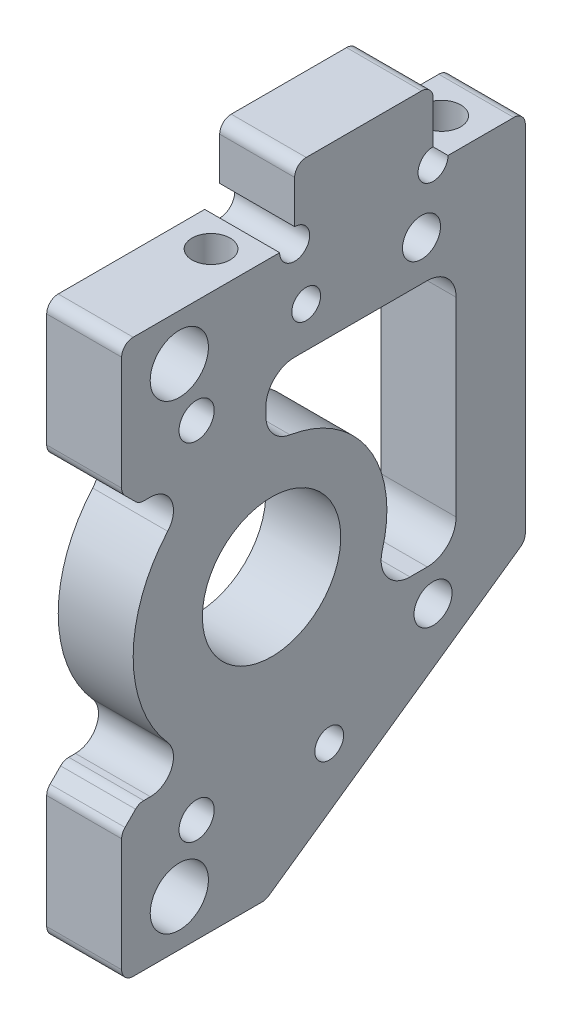
from build123d import *

# Parameters (mm, degrees)
SKETCH_1_R             = 6
SKETCH_1_R_2           = 1.525
SKETCH_1_R_3           = 2.525
EXTRUDE_1_DEPTH        = 6.5
FILLET_R2_5_1_R        = 2.5
HOLE_WIZARD_M3_1_D     = 2.5
HOLE_WIZARD_M4_1_D     = 3.3
HOLE_WIZARD_M4_1_DEPTH = 7
HOLE_WIZARD_M4_1_TIP   = 0.991420021
HOLE_WIZARD_M4_2_D     = 3.3
CHAMFER_C1_5_1_SIZE    = 1.5
FILLET_R1_2_R          = 1


with BuildPart() as part:
    # 草图1 → 凸台-拉伸1 (new body)
    with BuildSketch(Plane(origin=(0, 0, 0), x_dir=(0, 0, -1), z_dir=(1, 0, 0))):
        with BuildLine():
            Line((-13, 24), (-13, 11.25))
            Line((-13, 11.25), (-10.508924778, 11.25))
            ThreePointArc((-10.508924778, 11.25), (-8.68644609, 10.073754471), (-9.00764981, 7.928571429))
            ThreePointArc((-9.00764981, 7.928571429), (-12, 0), (-9.00764981, -7.928571429))
            ThreePointArc((-9.00764981, -7.928571429), (-8.68644609, -10.073754471), (-10.508924778, -11.25))
            Line((-10.508924778, -11.25), (-13, -11.25))
            Line((-13, -11.25), (-13, -24))
            Line((-13, -24), (-0.5, -24))
            Line((-0.5, -24), (22, -8.24533039))
            Line((22, -8.24533039), (22, 24))
            Line((22, 24), (15.3, 24))
            ThreePointArc((15.3, 24), (13.080761184, 23.080761184), (14, 25.3))
            Line((14, 25.3), (14, 30))
            Line((14, 30), (2, 30))
            Line((2, 30), (2, 25.3))
            ThreePointArc((2, 25.3), (2.919238816, 23.080761184), (0.7, 24))
            Line((0.7, 24), (-13, 24))
        make_face()
        with Locations(Location((0, 0, 0), (0, 0, 180))):
            Circle(SKETCH_1_R, mode=Mode.SUBTRACT)
        with Locations(Location((-6.5, 15, 0), (0, 0, 180))):
            Circle(SKETCH_1_R_2, mode=Mode.SUBTRACT)
        with Locations(Location((-8, 20, 0), (0, 0, 180))):
            Circle(SKETCH_1_R_3, mode=Mode.SUBTRACT)
        with Locations(Location((-6.5, -15, 0), (0, 0, 180))):
            Circle(SKETCH_1_R_2, mode=Mode.SUBTRACT)
        with Locations(Location((-8, -20, 0), (0, 0, 180))):
            Circle(SKETCH_1_R_3, mode=Mode.SUBTRACT)
        with BuildLine():
            Line((-0.5, 9.987492178), (-0.5, 15.5))
            Line((-0.5, 15.5), (16, 15.5))
            Line((16, 15.5), (16, -6))
            Line((16, -6), (8, -6))
            ThreePointArc((8, -6), (8.829636263, 4.694414071), (-0.5, 9.987492178))
        make_face(mode=Mode.SUBTRACT)
    extrude(amount=EXTRUDE_1_DEPTH)

    # R2.5 圆角1
    fillet_r2_5_1_edges = [part.edges().sort_by_distance(p)[0] for p in [
        (3.25, -6, -16),
        (3.25, 15.5, -16),
        (3.25, 15.5, 0.5),
        (3.25, 9.987492178, 0.5),
        (3.25, -6, -8),
    ]]
    fillet(fillet_r2_5_1_edges, radius=FILLET_R2_5_1_R)

    # M3 螺纹孔1 (through all)
    with Locations(Plane(origin=(6.5, 0, 0), x_dir=(0, 0, -1), z_dir=(1, 0, 0))):
        with Locations((5, -15), (3, 19)):
            Hole(HOLE_WIZARD_M3_1_D / 2)

    # M4 螺纹孔1
    with Locations(Plane(origin=(0, 24, 0), x_dir=(1, 0, 0), z_dir=(0, 1, 0))):
        with Locations((3.25, -2), (3.25, 18)):
            Hole(HOLE_WIZARD_M4_1_D / 2, depth=HOLE_WIZARD_M4_1_DEPTH)
            with Locations((0, 0, -(HOLE_WIZARD_M4_1_DEPTH + HOLE_WIZARD_M4_1_TIP / 2))):  # 118° drill point
                Cone(0, HOLE_WIZARD_M4_1_D / 2, HOLE_WIZARD_M4_1_TIP, mode=Mode.SUBTRACT)

    # M4 螺纹孔2 (through all)
    with Locations(Plane(origin=(6.5, 0, 0), x_dir=(0, 0, -1), z_dir=(1, 0, 0))):
        with Locations((14, -9), (13, 19)):
            Hole(HOLE_WIZARD_M4_2_D / 2)

    # C1.5 倒角1
    chamfer_c1_5_1_edges = [part.edges().sort_by_distance(p)[0] for p in [
        (3.25, -11.25, 13),
        (3.25, 11.25, 13),
    ]]
    chamfer(chamfer_c1_5_1_edges, length=CHAMFER_C1_5_1_SIZE)

    # R1 圆角2
    fillet_r1_2_edges = [part.edges().sort_by_distance(p)[0] for p in [
        (3.25, -12.75, 13),
        (3.25, -11.25, 11.5),
        (3.25, 11.25, 11.5),
        (3.25, 12.75, 13),
        (3.25, 30, -2),
        (3.25, 30, -14),
        (3.25, 24, -22),
        (3.25, -8.24533039, -22),
        (3.25, -24, 0.5),
        (3.25, -24, 13),
        (3.25, 24, 13),
    ]]
    fillet(fillet_r1_2_edges, radius=FILLET_R1_2_R)


solid = part.part
